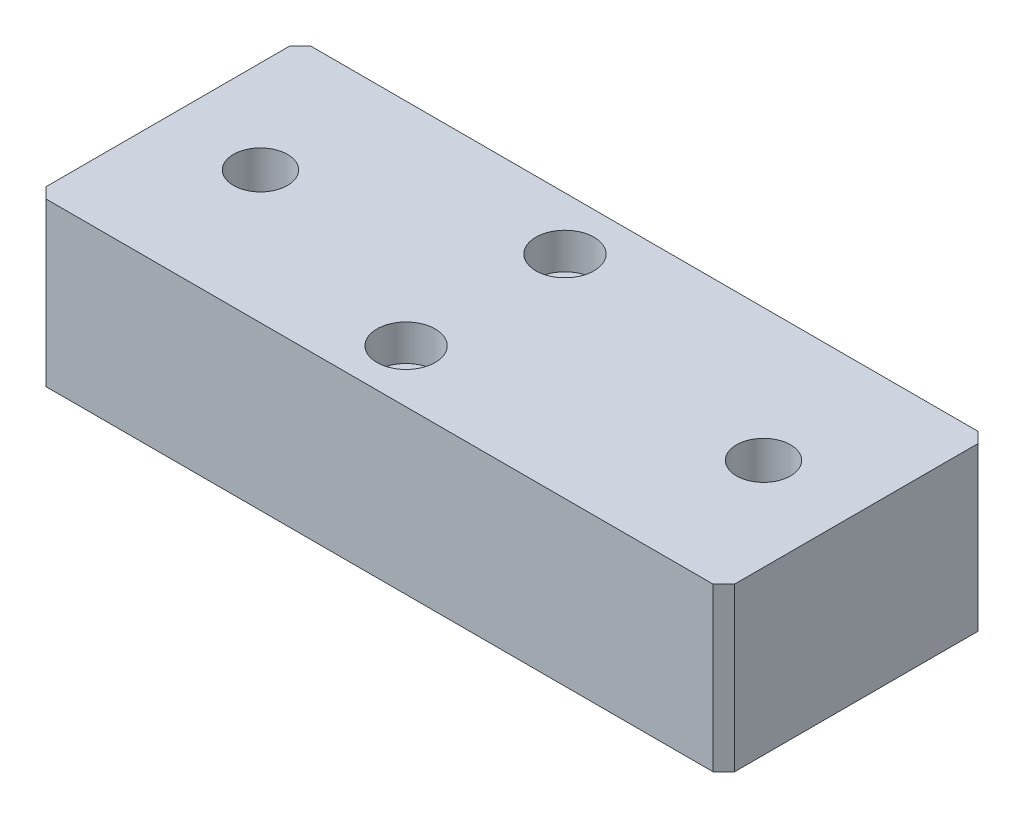
from build123d import *

# Parameters (mm, degrees)
SKETCH_1_W                = 130
SKETCH_1_H                = 50
EXTRUDE_1_DEPTH           = 15.35
CHAMFER_1_SIZE            = 2
HOLE_WIZARD_M12_1_D       = 10.2
HOLE_WIZARD_1_D           = 6.6
HOLE_WIZARD_1_CBORE_D     = 11
HOLE_WIZARD_1_CBORE_DEPTH = 6.8


with BuildPart() as part:
    # 草图1 → 凸台-拉伸1 (new, symmetric)
    with BuildSketch(Plane(origin=(0, 0, 0), x_dir=(1, 0, 0), z_dir=(0, 1, 0))):
        Rectangle(SKETCH_1_W, SKETCH_1_H)
    extrude(amount=EXTRUDE_1_DEPTH, both=True)

    # 倒角1
    chamfer_1_edges = [part.edges().sort_by_distance(p)[0] for p in [
        (65, 0, 25),
        (-65, 0, 25),
        (-65, 0, -25),
        (65, 0, -25),
    ]]
    chamfer(chamfer_1_edges, length=CHAMFER_1_SIZE)

    # M12 螺纹孔1 (through all)
    with Locations(Plane(origin=(0, 15.35, 0), x_dir=(1, 0, 0), z_dir=(0, 1, 0))):
        with Locations((-47.5, 0), (47.5, 0)):
            Hole(HOLE_WIZARD_M12_1_D / 2)

    # 打孔尺寸(%根据)内六角圆柱头螺钉的类型1 (through all)
    with Locations(Plane(origin=(0, 15.35, 0), x_dir=(1, 0, 0), z_dir=(0, 1, 0))):
        with Locations((-5, -15), (-5, 15)):
            CounterBoreHole(HOLE_WIZARD_1_D / 2, HOLE_WIZARD_1_CBORE_D / 2, HOLE_WIZARD_1_CBORE_DEPTH)


solid = part.part
